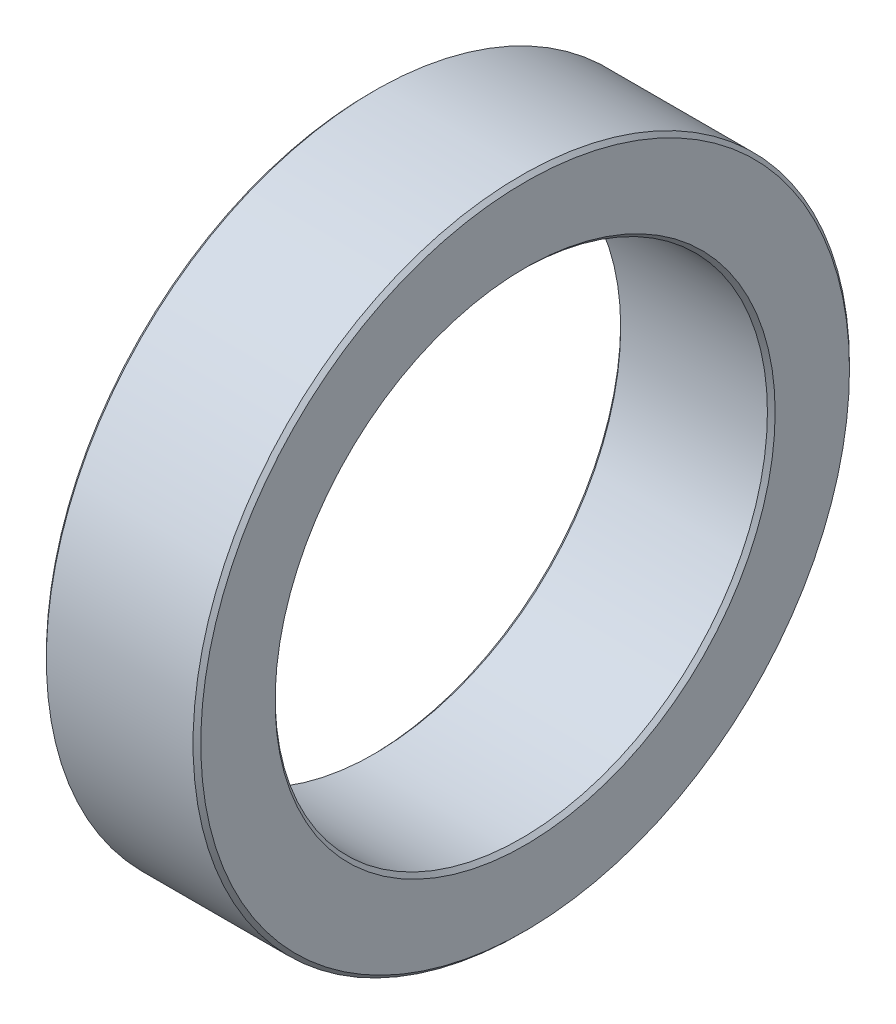
SolidWorks part; units mm, degrees
material "S45C"
ref_plane "Front Plane" through (0, 0, 0) normal (0, 0, 1) x (1, 0, 0)
ref_plane "Top Plane" through (0, 0, 0) normal (0, 1, 0) x (1, 0, 0)
ref_plane "Right Plane" through (0, 0, 0) normal (1, 0, 0) x (0, 0, -1)
sketch "Sketch1" plane through (0, 0, 0) normal (1, 0, 0) x (0, 0, -1)
  circle A0 centre (0, 0) radius 17
  circle A1 centre (0, 0) radius 12.75
  dimension "D1" = 34
  dimension "D2" = 25.5
extrude "Boss-Extrude1" add sketch "Sketch1" along normal mid plane 8
chamfer "Chamfer1" distance 0.2 angle 45 4 edges at (4, 0, -17) (4, 0, -12.75) (-4, 0, -17) (-4, 0, -12.75)
